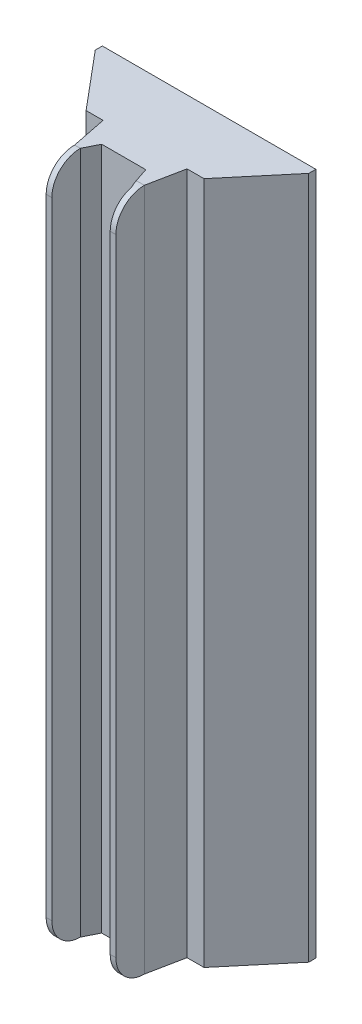
SolidWorks part; units mm, degrees
material "AISI 304"
ref_plane "Front Plane" through (0, 0, 0) normal (0, 0, 1) x (1, 0, 0)
ref_plane "Top Plane" through (0, 0, 0) normal (0, 1, 0) x (1, 0, 0)
ref_plane "Right Plane" through (0, 0, 0) normal (1, 0, 0) x (0, 0, -1)
sketch "Sketch1" plane through (0, 0, 0) normal (0, 1, 0) x (1, 0, 0)
  line L0 (0, 0) -> (0, -50000) construction
  line L1 (-7.5, 2.25) -> (7.5, 2.25)
  line L2 (-7.5, 2.25) -> (-7.5, -2.25)
  line L3 (-7.5, -2.25) -> (-2.45, -2.25)
  line L4 (7.5, 2.25) -> (7.5, -2.25)
  line L5 (-7.5, 2.25) -> (7.5, -2.25) construction
  line L6 (-7.5, -2.25) -> (7.5, 2.25) construction
  line L7 (2.45, -2.25) -> (7.5, -2.25)
  line L8 (-2.45, -6.75) -> (-2.05, -6.75)
  line L9 (-2.45, -6.75) -> (-2.45, -2.25)
  line L11 (2.45, -6.75) -> (2.45, -2.25)
  line L12 (-2.45, -6.75) -> (2.45, -2.25) construction
  line L13 (-2.45, -2.25) -> (2.45, -6.75) construction
  line L14 (2.05, -6.75) -> (2.45, -6.75)
  line L15 (-2.05, -6.75) -> (-2.05, -3.75)
  line L16 (-2.05, -3.75) -> (2.05, -3.75)
  line L17 (2.05, -6.75) -> (2.05, -3.75)
  line L18 (-3.1704, -25.288) -> (2.05, -3.75) construction
  line L19 (-2.05, -3.75) -> (3.275, -25.7195) construction
  point P0 (0, 0)
  point P8 (0, -4.5)
  point P13 (0, -12.2077)
  dimension "D1" = 15
  dimension "D2" = 9
  dimension "D3" = 4.9
  dimension "D4" = 0.4
  dimension "D5" = 3
  dimension "D6" = 4.5
extrude "Boss-Extrude1" add sketch "Sketch1" along normal blind 48
chamfer "Chamfer1" distance 1 distance2 0.5 1 edges at (-2.05, 24, 3.75)
chamfer "Chamfer2" distance 0.5 distance2 1.5 1 edges at (2.05, 24, 3.75)
chamfer "Chamfer3" distance 0.5 distance2 2.5 1 edges at (-2.45, 24, 2.25)
chamfer "Chamfer4" distance 2.5 distance2 0.5 1 edges at (2.45, 24, 2.25)
chamfer "Chamfer5" distance 4 angle 40 1 edges at (-7.5, 24, 2.25)
chamfer "Chamfer6" distance 4 angle 40 1 edges at (7.5, 24, 2.25)
fillet "Fillet1" radius 2 4 edges at (-2.25, 0, 6.75) (2.25, 0, 6.75) (-2.25, 48, 6.75) (2.25, 48, 6.75)
